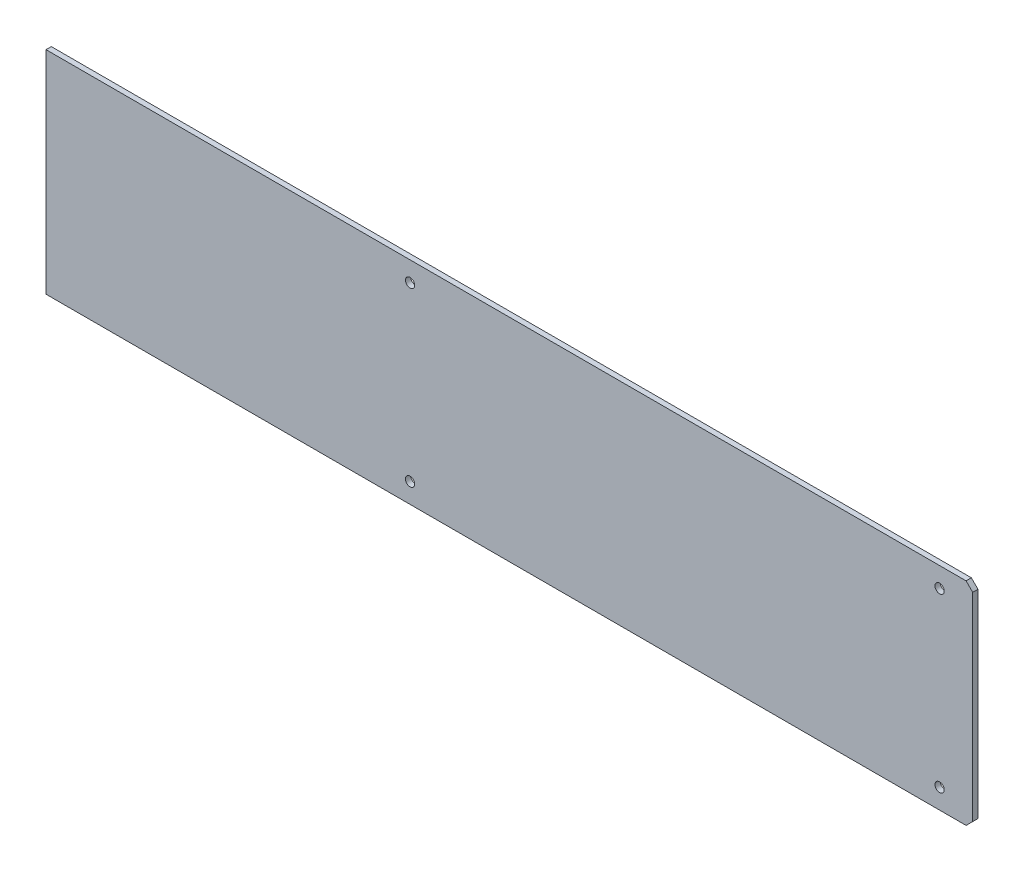
from build123d import *

# Parameters (mm, degrees)
SKETCH1_W           = 700
SKETCH1_H           = 160
BOSS_EXTRUDE1_DEPTH = 4
SKETCH2_R           = 3.5
CUT_EXTRUDE1_DEPTH  = 4
CHAMFER1_SIZE       = 5


with BuildPart() as part:
    # Sketch1 → Boss-Extrude1 (new body)
    with BuildSketch(Plane.XY):
        Rectangle(SKETCH1_W, SKETCH1_H)
    extrude(amount=BOSS_EXTRUDE1_DEPTH)

    # Sketch2 → Cut-Extrude1 (cut)
    with BuildSketch(Plane.XY.offset(4)):
        with Locations((-75, 65)):
            Circle(SKETCH2_R)
        with Locations((325, 65)):
            Circle(SKETCH2_R)
        with Locations((325, -65)):
            Circle(SKETCH2_R)
        with Locations((-75, -65)):
            Circle(SKETCH2_R)
    extrude(amount=-CUT_EXTRUDE1_DEPTH, mode=Mode.SUBTRACT)

    # Chamfer1
    chamfer1_edges = [part.edges().sort_by_distance(p)[0] for p in [
        (350, 80, 2),
        (350, -80, 2),
    ]]
    chamfer(chamfer1_edges, length=CHAMFER1_SIZE)


solid = part.part
